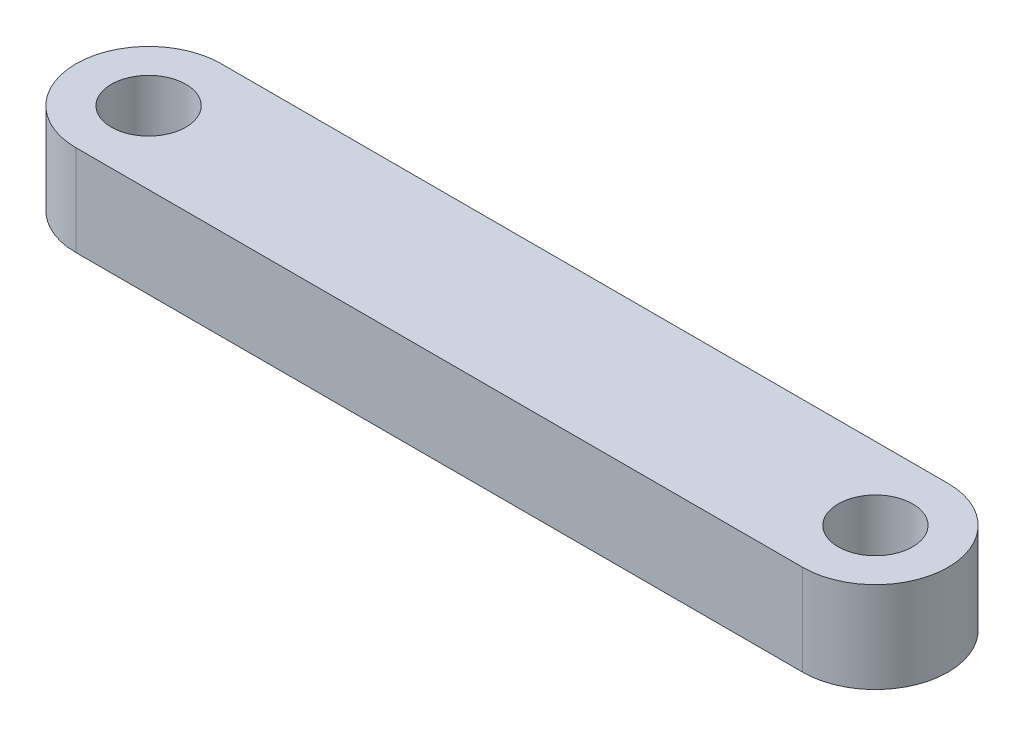
SolidWorks part; units mm, degrees
material "ABS"
ref_plane "Front Plane" through (0, 0, 0) normal (0, 0, 1) x (1, 0, 0)
ref_plane "Top Plane" through (0, 0, 0) normal (0, 1, 0) x (1, 0, 0)
ref_plane "Right Plane" through (0, 0, 0) normal (1, 0, 0) x (0, 0, -1)
sketch "Sketch1" plane through (0, 0, 0) normal (0, 1, 0) x (1, 0, 0)
  line L0 (0, 5.08) -> (50.8, 5.08)
  line L1 (0, -5.08) -> (50.8, -5.08)
  line L2 (0, 0) -> (17.9912, 0) construction
  circle A0 centre (0, 0) radius 2.9
  circle A1 centre (0, 0) radius 5.08 construction
  arc A2 (0, -5.08) -> (0, 5.08) centre (0, 0) cw
  circle A3 centre (50.8, 0) radius 2.9
  circle A4 centre (50.8, 0) radius 5.08 construction
  arc A5 (50.8, 5.08) -> (50.8, -5.08) centre (50.8, 0) cw
  point P8 (-5.08, 0)
  point P14 (55.88, 0)
  dimension "D1" = 5.8
  dimension "D2" = 10.16
  dimension "D4" = 50.8
extrude "Boss-Extrude1" add sketch "Sketch1" along normal blind 6.35
sketch "Sketch2" plane through (0, 6.35, 0) normal (0, 1, 0) x (1, 0, 0)
  circle A0 centre (0, 0) radius 2.6035
  circle A1 centre (0, 0) radius 2.9
  circle A2 centre (50.8, 0) radius 2.9
  circle A3 centre (50.8, 0) radius 2.6035
  circle A4 centre (0, 0) radius 2.9 construction
  circle A5 centre (50.8, 0) radius 2.9 construction
  dimension "D1" = 5.207
extrude "Boss-Extrude2" add sketch "Sketch2" against normal up to surface (6.35 mm away) up to face at (0, 0, 2.9)
